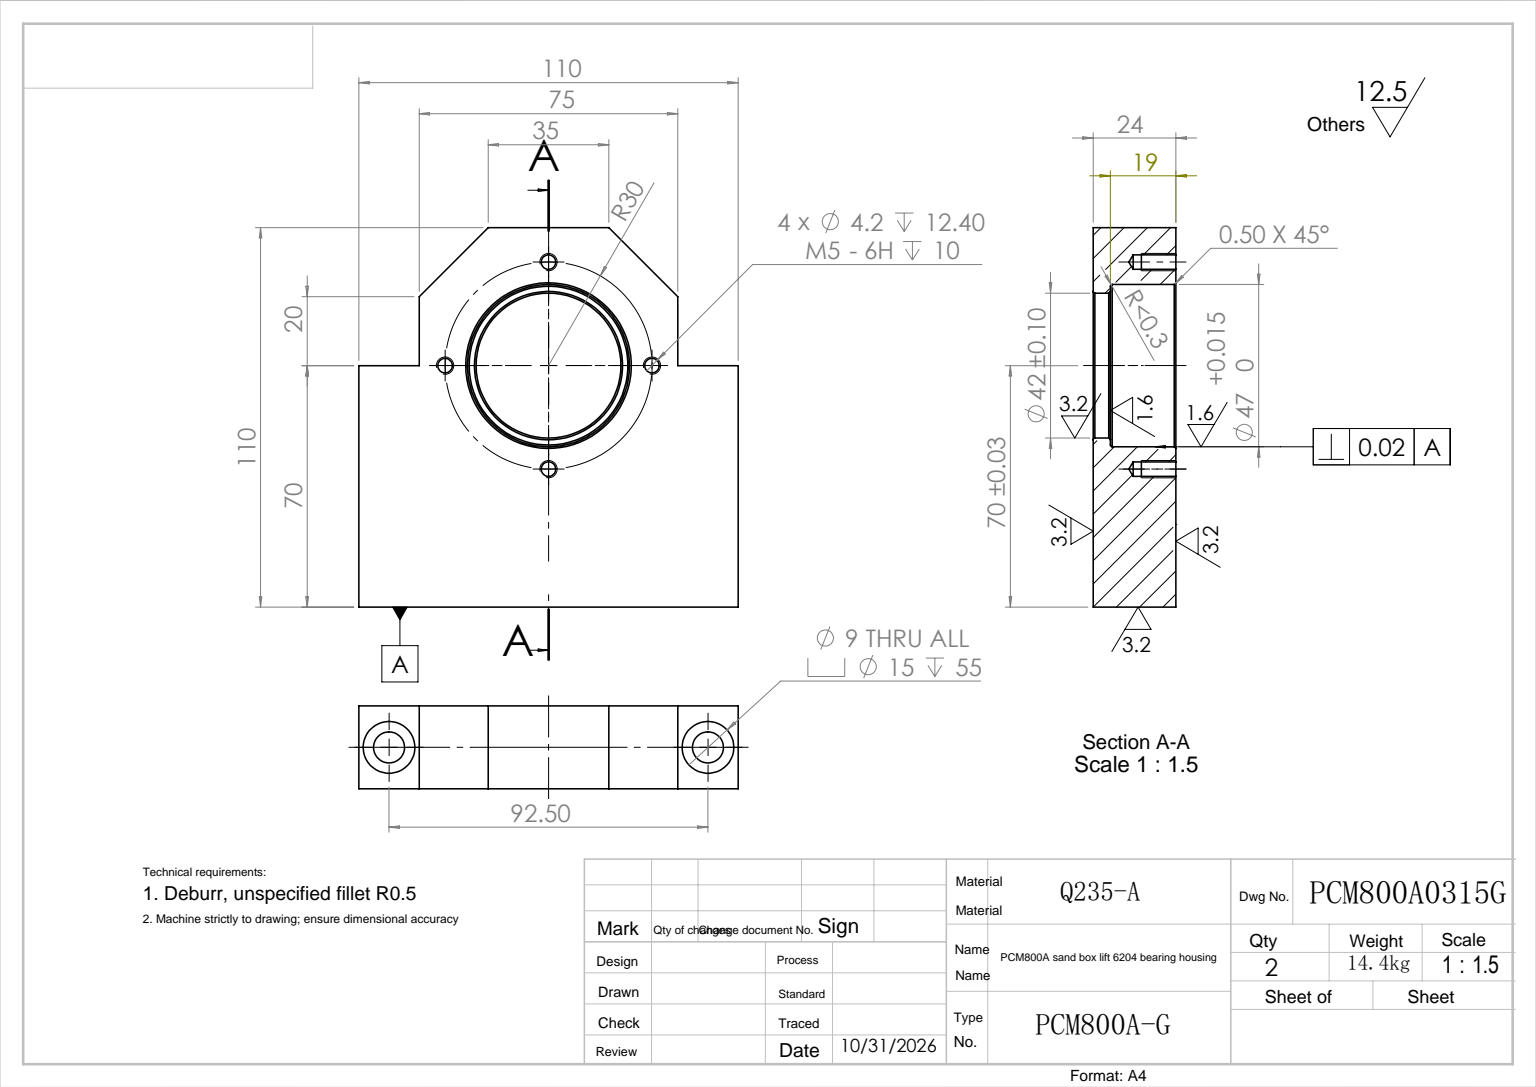
SolidWorks part; units mm, degrees
ref_plane "前视基准面" through (0, 0, 0) normal (0, 0, 1) x (1, 0, 0)
ref_plane "上视基准面" through (0, 0, 0) normal (0, 1, 0) x (1, 0, 0)
ref_plane "右视基准面" through (0, 0, 0) normal (1, 0, 0) x (0, 0, -1)
sketch "草图1" plane through (0, 0, 0) normal (0, 1, 0) x (1, 0, 0)
  line L1 (0, 0) -> (110, 0)
  line L2 (0, 0) -> (0, 24)
  line L3 (0, 24) -> (110, 24)
  line L4 (110, 0) -> (110, 24)
  dimension "D1" = 24
  dimension "D2" = 110
extrude "拉伸1" add sketch "草图1" along normal blind 110
sketch "草图2" plane through (0, 0, 0) normal (0, 0, 1) x (1, 0, 0)
  line L0 (0, 70) -> (110, 70) construction
  line L1 (0, 110) -> (0, 0) construction
  line L2 (110, 110) -> (110, 0) construction
  line L3 (55, 70) -> (55, 0) construction
  line L4 (0, 0) -> (110, 0) construction
  circle A0 centre (55, 70) radius 21
  dimension "D1" = 70
extrude "切除-拉伸1" cut sketch "草图2" against normal blind 5
sketch "草图3" plane through (0, 0, -5) normal (0, 0, 1) x (1, 0, 0)
  circle A0 centre (55, 70) radius 23.5
extrude "切除-拉伸2" cut sketch "草图3" against normal blind 19
sketch "草图4" plane through (0, 0, -24) normal (0, 0, -1) x (-1, 0, 0)
  circle A0 centre (-55, 70) radius 37.5 construction
sketch "草图5" plane through (0, 0, -24) normal (0, 0, -1) x (-1, 0, 0)
  line L0 (-92.5, 70) -> (-110, 70)
  line L1 (-110, 110) -> (-110, 0) construction
  line L2 (-92.5, 70) -> (-92.5, 110)
  line L3 (-110, 110) -> (0, 110) construction
  line L4 (-17.5, 70) -> (-17.5, 110)
  line L5 (-17.5, 70) -> (0, 70)
  line L6 (0, 110) -> (0, 0) construction
  line L7 (-92.5, 110) -> (-110, 110)
  line L8 (-110, 110) -> (-110, 70)
  line L9 (-17.5, 110) -> (0, 110)
  line L10 (0, 110) -> (0, 70)
  circle A0 centre (-55, 70) radius 37.5 construction
  dimension "D1" = 17.5
  dimension "D2" = 17.5
extrude "切除-拉伸3" cut sketch "草图5" against normal through all
chamfer "倒角1" distance 20 angle 45 2 edges at (17.5, 110, -12) (92.5, 110, -12)
sketch "草图6" plane through (0, 0, -24) normal (0, 0, -1) x (-1, 0, 0)
  line L0 (-55, 100) -> (-55, 103.2162) construction
  line L1 (-25, 70) -> (-22.6181, 70) construction
  line L2 (-85, 70) -> (-87.4331, 70) construction
  line L3 (-55, 40) -> (-55, 36.7367) construction
  circle A0 centre (-55, 70) radius 30 construction
hole_wizard "M5 螺纹孔1" positions "3D草图1" profile "草图7" tap size "M5" standard "GB"
sketch3d "3D草图1"
  point P0 (55, 100, -24)
  point P3 (85, 70, -24)
  point P6 (55, 40, -24)
  point P9 (25, 70, -24)
sketch "草图7" plane through (55, 100, -24) normal (1, 0, 0) x (0, 1, 0)
  line L0 (0, 0) -> (0, 13.6618)
  line L1 (0, 13.6618) -> (2.1, 12.4)
  line L2 (2.1, 12.4) -> (2.1, 0)
  line L5 (2.1, 0) -> (0, 0)
  line L10 (0, 13.6618) -> (-2.1, 12.4) construction
  line L11 (0, -6.35) -> (0, 107.95) construction
  dimension "蹟恇謂郰芛眻噤" = 4.2
  dimension "蹟恇謂郰芛旮僅" = 12.4
  dimension "絳芛褒僅" = 118
cosmetic thread "孔螺蚊线1" parameters "D1"=10, "D2"=5
cosmetic thread "孔螺蚊线2" parameters "D1"=10, "D2"=5
cosmetic thread "孔螺蚊线3" parameters "D1"=10, "D2"=5
cosmetic thread "孔螺蚊线4" parameters "D1"=10, "D2"=5
hole_wizard "打孔尺寸根据内六角圆柱头螺钉的类型1" positions "3D草图2" profile "草图8" counterbore size "M8" standard "GB" end condition through all
sketch3d "3D草图2"
  line L0 (0, 70, 0) -> (0, 70, -24) construction
  line L1 (17.5, 70, -24) -> (0, 70, -24) construction
  line L2 (110, 70, -24) -> (92.5, 70, -24) construction
  line L3 (110, 70, 0) -> (110, 70, -24) construction
  point P0 (8.75, 70, -12)
  point P2 (101.25, 70, -12)
  dimension "D1" = 8.75
  dimension "D2" = 12
  dimension "D3" = 12
  dimension "D4" = 8.75
sketch "草图8" plane through (8.75, 70, -12) normal (1, 0, 0) x (0, 0, 1)
  line L0 (0, 0) -> (0, 70)
  line L1 (0, 70) -> (4.5, 70)
  line L3 (4.5, 70) -> (4.5, 55)
  line L4 (4.5, 55) -> (7.5, 55)
  line L5 (7.5, 55) -> (7.5, 0)
  line L7 (7.5, 0) -> (0, 0)
  line L11 (0, -6.35) -> (0, 107.95) construction
  dimension "通孔孔直径" = 9
  dimension "通孔孔深度" = 70
  dimension "柱形沉头孔直径" = 15
  dimension "柱形沉头孔深度" = 55
fillet "圆角2" radius 0.5 3 edges at (78.5, 70, -5) (76, 70, 0) (76, 70, -5)
chamfer "倒角2" distance 0.5 angle 45 1 edges at (78.5, 70, -24)
